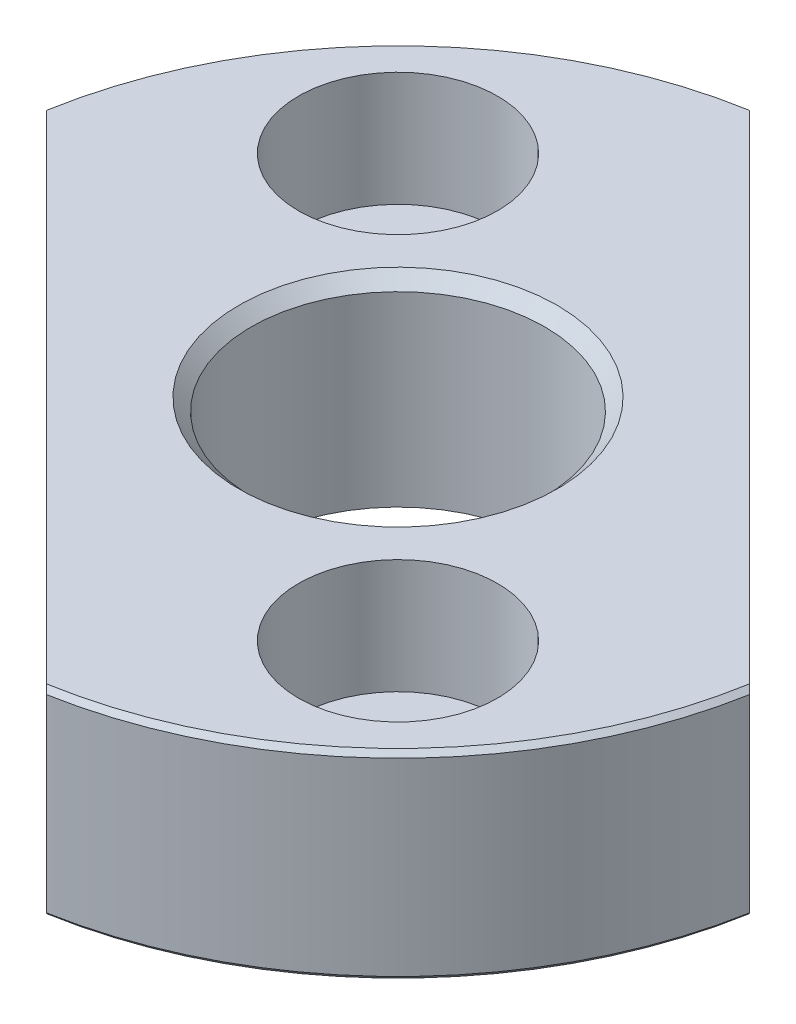
SolidWorks part; units mm, degrees
material "AISI 类型 316L 不锈钢"
ref_plane "Front Plane" through (0, 0, 0) normal (0, 0, 1) x (1, 0, 0)
ref_plane "Top Plane" through (0, 0, 0) normal (0, 1, 0) x (1, 0, 0)
ref_plane "Right Plane" through (0, 0, 0) normal (1, 0, 0) x (0, 0, -1)
sketch "Sketch2" plane through (0, 0, 0) normal (0, 0, 1) x (1, 0, 0)
  line L0 (0, 0) -> (0, 24) construction
  line L1 (0, 24) -> (-17.5, 24)
  line L2 (-17.5, 24) -> (-17.5, 16)
  line L3 (-17.5, 16) -> (-6.75, 16)
  line L4 (-6.75, 16) -> (-6.75, 0)
  line L5 (-6.75, 0) -> (0, 0)
  line L6 (0, 0) -> (0, 24)
  dimension "D1" = 35
  dimension "D2" = 13.5
  dimension "D3" = 16
  dimension "D4" = 8
revolve "Revolve1" add sketch "Sketch2" angle 360 about L0
hole_wizard "G1/4 Tapped Hole1" positions "3DSketch1" profile "Sketch4" tap size "G1/4" standard "GB" end condition up to next
sketch3d "3DSketch1"
  line L0 (0, 24, 0) -> (0, 16, 0) construction
  point P0 (0, 24, 0)
sketch "Sketch4" plane through (0, 24, 0) normal (1, 0, 0) x (0, 0, 1)
  line L0 (0, 0) -> (0, 24)
  line L1 (0, 24) -> (5.9, 24)
  line L2 (5.9, 24) -> (5.9, 0)
  line L5 (5.9, 0) -> (0, 0)
  line L11 (0, -6.35) -> (0, 107.95) construction
  dimension "通孔螺纹孔钻头直径" = 11.8
  dimension "通孔螺纹孔钻头深度" = 24
cosmetic thread "Cosmetic Thread 1" parameters "D2"=13.157
sketch "Sketch5" plane through (0, 24, 0) normal (0, 1, 0) x (1, 0, 0)
  line L0 (0, 12) -> (0, -12) construction
  line L1 (12, 0) -> (-12, 0) construction
  line L2 (0, 0) -> (-8.4853, 8.4853) construction
  line L3 (0, 0) -> (8.4853, -8.4853) construction
  circle A0 centre (0, 0) radius 12 construction
  dimension "D1" = 24
  dimension "D2" = 45
hole_wizard "Hole Size (% based on) Socket Head Cap Screw Type 1" positions "3DSketch2" profile "Sketch6" counterbore size "M4" standard "GB" end condition up to next
sketch3d "3DSketch2"
  point P13 (-8.4853, 24, -8.4853)
  point P16 (8.4853, 24, 8.4853)
sketch "Sketch6" plane through (-8.4853, 24, -8.4853) normal (1, 0, 0) x (0, 0, 1)
  line L0 (0, 0) -> (0, 8)
  line L1 (0, 8) -> (2.4, 8)
  line L3 (2.4, 8) -> (2.4, 4.6)
  line L4 (2.4, 4.6) -> (4, 4.6)
  line L5 (4, 4.6) -> (4, 0)
  line L7 (4, 0) -> (0, 0)
  line L11 (0, -6.35) -> (0, 107.95) construction
  dimension "通孔孔直径" = 4.8
  dimension "通孔孔深度" = 8
  dimension "柱形沉头孔直径" = 8
  dimension "柱形沉头孔深度" = 4.6
fillet "Fillet1" radius 0.2 1 edges at (0, 16, -6.75)
chamfer "Chamfer1" distance 0.2 angle 45 3 edges at (0, 0, -6.75) (0, 24, -17.5) (0, 16, -17.5)
chamfer "Chamfer2" distance 0.5 angle 45 2 edges at (0, 0, 5.9) (0, 24, 5.9)
sketch "Sketch7" plane through (0, 24, 0) normal (0, 1, 0) x (1, 0, 0)
  line L0 (0, 0) -> (12.2329, 12.2329) construction
  line L1 (0, 0) -> (17.3, 0) construction
  line L2 (-3.084, 17.2261) -> (17.2261, -3.084)
  line L3 (0, 0) -> (12.2329, -12.2329) construction
  line L4 (0, 12) -> (0, -12) construction
  line L5 (-17.2261, 3.084) -> (3.084, -17.2261)
  circle A0 centre (0, 0) radius 17.3 construction
  circle A1 centre (0, 0) radius 17.5 construction
  circle A2 centre (0, 0) radius 17.5
  point P9 (7.0711, 7.0711)
  circle M7 centre (0, 0) radius 17.3
  dimension "D1" = 45
  dimension "D2" = 45
  dimension "D3" = 10
extrude "Cut-Extrude1" cut sketch "Sketch7" against normal through all contours L5 M7 | L2 M7 | L5 A2 M7 | L2 A2 M7
sketch "Sketch8" plane through (0, 16, 0) normal (0, -1, 0) x (1, 0, 0)
  circle A0 centre (0, 0) radius 15
  dimension "D1" = 30
extrude "Cut-Extrude2" cut sketch "Sketch8" along normal through all
